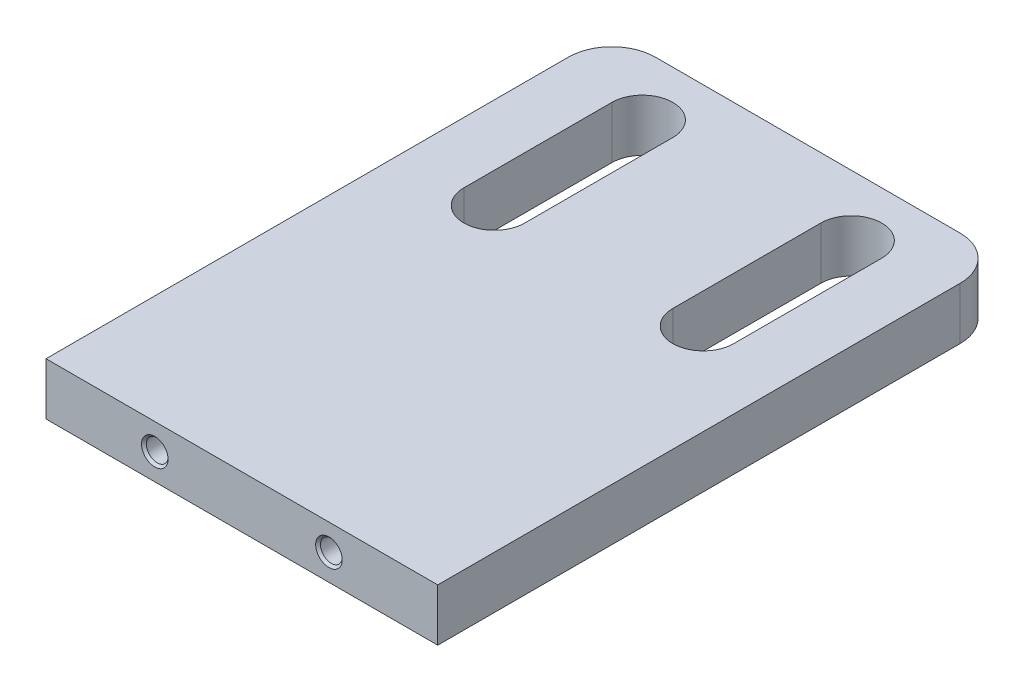
SolidWorks part; units mm, degrees
material "SPCC"
ref_plane "Front Plane" through (0, 0, 0) normal (0, 0, 1) x (1, 0, 0)
ref_plane "Top Plane" through (0, 0, 0) normal (0, 1, 0) x (1, 0, 0)
ref_plane "Right Plane" through (0, 0, 0) normal (1, 0, 0) x (0, 0, -1)
sketch "Sketch1" plane through (0, 0, 0) normal (0, 1, 0) x (1, 0, 0)
  line L1 (22.5, -32.5) -> (-22.5, -32.5)
  line L2 (22.5, -32.5) -> (22.5, 32.5)
  line L3 (22.5, 32.5) -> (-22.5, 32.5)
  line L4 (-22.5, -32.5) -> (-22.5, 32.5)
  line L5 (22.5, -32.5) -> (-22.5, 32.5) construction
  line L6 (22.5, 32.5) -> (-22.5, -32.5) construction
  point P0 (0, 0)
  dimension "D1" = 45
  dimension "D2" = 65
extrude "Boss-Extrude1" add sketch "Sketch1" along normal blind 6
sketch "Sketch6" plane through (0, 6, 0) normal (0, 1, 0) x (1, 0, 0)
  line L0 (0, 0) -> (0, 25.0024) construction
  line L1 (-12, 25.5) -> (-12, 8.5) construction
  line L2 (-8.5, 25.5) -> (-8.5, 8.5)
  line L3 (-15.5, 25.5) -> (-15.5, 8.5)
  line L4 (12, 25.5) -> (12, 8.5) construction
  line L5 (8.5, 25.5) -> (8.5, 8.5)
  line L6 (15.5, 25.5) -> (15.5, 8.5)
  line L7 (22.5, 32.5) -> (-22.5, 32.5) construction
  arc A0 (-8.5, 25.5) -> (-15.5, 25.5) centre (-12, 25.5) ccw
  arc A1 (-15.5, 8.5) -> (-8.5, 8.5) centre (-12, 8.5) ccw
  arc A2 (8.5, 25.5) -> (15.5, 25.5) centre (12, 25.5) cw
  arc A3 (15.5, 8.5) -> (8.5, 8.5) centre (12, 8.5) cw
  point P5 (-12, 17)
  point P12 (12, 17)
  dimension "D1" = 7
  dimension "D2" = 17
  dimension "D3" = 7
  dimension "D4" = 17
extrude "Cut-Extrude1" cut sketch "Sketch6" against normal blind 6
fillet "Fillet2" radius 5 2 edges at (22.5, 3, -32.5) (-22.5, 3, -32.5)
hole_wizard "M3 Tapped Hole1" positions "Sketch9" profile "Sketch8" tap size "M3" standard "GB"
sketch "Sketch9" plane through (0, 0, 32.5) normal (0, 0, 1) x (1, 0, 0)
  line L0 (-10, 3) -> (10, 3) construction
  line L2 (0, 0) -> (0, 3) construction
  point P0 (-10, 3)
  point P2 (10, 3)
  dimension "D1" = 3
  dimension "D2" = 20
cosmetic thread "Hole thread line1" parameters "D1"=12, "D2"=3
cosmetic thread "Hole thread line2" parameters "D1"=12, "D2"=3
sketch "Sketch8" plane through (-10, 3, 32.5) normal (1, 0, 0) x (0, -1, 0)
  line L0 (0, 0) -> (0, 14.2511)
  line L1 (0, 14.2511) -> (1.25, 13.5)
  line L2 (1.25, 13.5) -> (1.25, 0.275)
  line L3 (1.25, 0.275) -> (1.525, 0)
  line L5 (1.525, 0) -> (0, 0)
  line L6 (-1.25, 0.275) -> (-1.525, 0) construction
  line L10 (0, 14.2511) -> (-1.25, 13.5) construction
  line L11 (0, -6.35) -> (0, 107.95) construction
  dimension "螺纹孔钻头直径" = 2.5
  dimension "螺纹孔钻头深度" = 13.5
  dimension "近端锥形沉头孔直径" = 3.05
  dimension "近端锥形沉头孔角度" = 90
  dimension "导头角度" = 118
